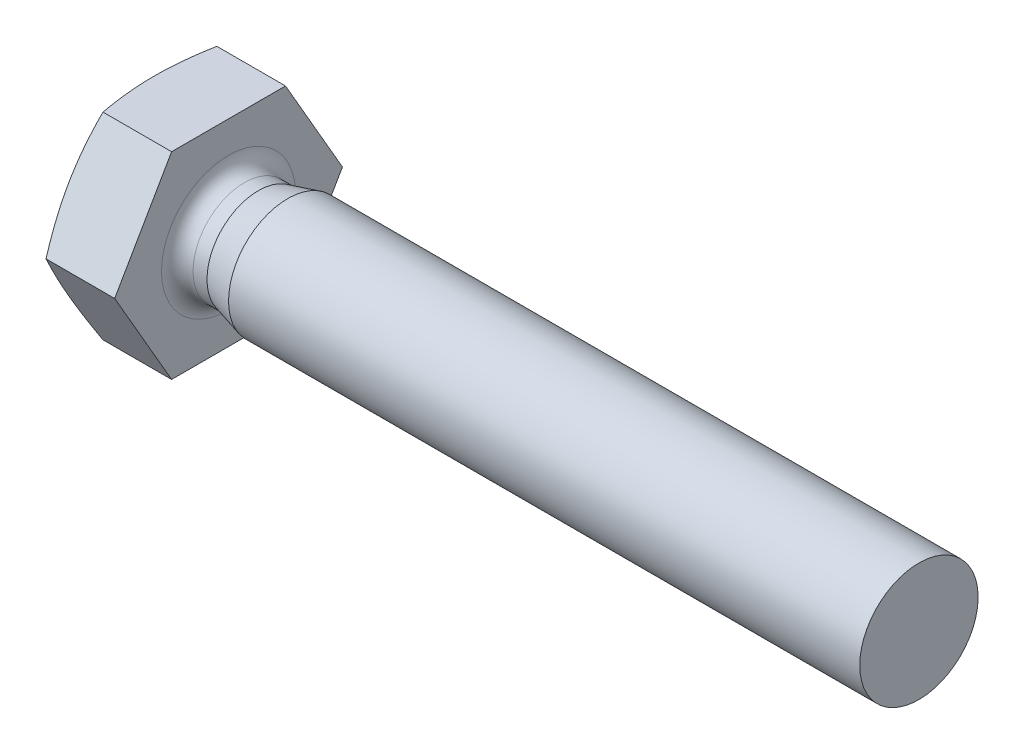
SolidWorks part; units mm, degrees
material "S45C"
ref_plane "Front" through (0, 0, 0) normal (0, 0, 1) x (1, 0, 0)
ref_plane "Top" through (0, 0, 0) normal (0, 1, 0) x (1, 0, 0)
ref_plane "Right" through (0, 0, 0) normal (1, 0, 0) x (0, 0, -1)
other "Configuration Table"
sketch "Sketch2" plane through (0, 0, 0) normal (1, 0, 0) x (0, 0, -1)
  line L1 (2.8868, -5) -> (5.7735, 0)
  line L2 (5.7735, 0) -> (2.8868, 5)
  line L3 (2.8868, 5) -> (-2.8868, 5)
  line L4 (-2.8868, 5) -> (-5.7735, 0)
  line L5 (-5.7735, 0) -> (-2.8868, -5)
  line L6 (-2.8868, -5) -> (2.8868, -5)
  circle A0 centre (0, 0) radius 5 construction
  dimension "s" = 10
extrude "BaseHead" add sketch "Sketch2" along normal blind 4
sketch "Sketch10" plane through (0, 0, 0) normal (0, 1, 0) x (1, 0, 0)
  line L0 (0, 0) -> (15.3195, 0) construction
  line L1 (4, 3.4) -> (4, 0)
  line L2 (4, 0) -> (39, 0)
  line L3 (4, 2.8868) -> (4, -2.8868) construction
  line L4 (7, 3) -> (39, 3)
  line L5 (39, 0) -> (39, 3)
  line L6 (4.8, 2.6) -> (5.5072, 2.6)
  line L7 (4, 5.7735) -> (4, 2.8868) construction
  line L8 (7, 3) -> (5.5072, 2.6)
  line L9 (4, 5.7735) -> (4, 2.8868) construction
  arc A0 (4, 3.4) -> (4.8, 2.6) centre (4.8, 3.4) ccw
revolve "Revolve1" add sketch "Sketch10" angle 360 about L0
cosmetic thread "ThreadCosmetic1" [suppressed] parameters "D2"=4.917
sketch "Sketch5" plane through (0, 0, 0) normal (0, 1, 0) x (1, 0, 0)
  line L0 (0, 5.7735) -> (0.5181, 5.7735)
  line L1 (0, 5.7735) -> (0, 2.8868) construction
  line L2 (0.5181, 5.7735) -> (0, 4.35)
  line L3 (4, 5.7735) -> (0, 5.7735) construction
  line L4 (0, 4.35) -> (0, 5.7735)
  line L5 (-0.3584, 0) -> (3.3946, 0) construction
revolve "HeadChamfer" cut sketch "Sketch5" angle 360 about L5
ref_plane "Plane1" through (1.4, 0, 0) normal (1, 0, 0) x (0, 0, -1)
sketch "Sketch6" plane through (0, 0, 0) normal (-1, 0, 0) x (0, 0, 1)
  circle A0 centre (0, 0) radius 4.35
extrude "Cut-Extrude1" cut sketch "Sketch6" against normal blind 1.4
sketch "Sketch7" plane through (0, 0, 0) normal (0, 1, 0) x (1, 0, 0)
  line L0 (1.4, 0) -> (6.7401, 0) construction
  line L1 (1.4, 4.35) -> (1.4, -4.35) construction
  line L2 (4.26, 0) -> (0.9, 3.642)
  line L4 (0.9, 3.642) -> (0.9, -3.642)
  line L5 (0.9, -3.642) -> (4.26, 0)
  line L7 (1.4, 3.1) -> (1.4, -3.1) construction
extrude "Cut-Extrude2" cut sketch "Sketch7" against normal mid plane 1.144
pattern_circular "CirPattern2" count 2 every 90 about axis through (0, 0, 0) along (1, 0, 0) of "Cut-Extrude2"
sketch "Sketch8" plane through (0, 0, 0) normal (0, 0, 1) x (1, 0, 0)
  line L0 (39, 2.531) -> (39.2708, 3)
  line L1 (39.2708, 3) -> (39.2708, 3.5415)
  line L2 (39.2708, 3.5415) -> (38.7293, 3.5415)
  line L3 (38.7293, 3.5415) -> (38.7293, 3)
  line L4 (38.7293, 3) -> (39, 2.531)
  line L5 (14.8, 0) -> (0, 0) construction
  line L6 (39, -3) -> (39, 3) construction
  line L7 (39, 3) -> (7, 3) construction
revolve "Cut-Revolve10" [suppressed] cut sketch "Sketch8" angle 360 about L5
pattern_linear "LPattern10" [suppressed] count 49 along (1, 0, 0)
equation "\"D1@Sketch6\" = \"dw@Sketch5\""
equation "\"D1@Cut-Extrude1\" = \"k@BaseHead\" - \"k1@Plane1\""
equation "\"t@Cut-Extrude2\" = 0.4 * \"h@Sketch7\""
equation "\"D1@Sketch8\" =  ( \"d@Sketch10\" - \"D2@ThreadCosmetic1\" )  / 2"
equation "\"pitch@LPattern10\" = \"D1@Sketch8\" * 1.2"
equation "\"D1@LPattern10\" =  ( \"l@Sketch10\" - \"a@Sketch10\" )  / \"pitch@LPattern10\""
